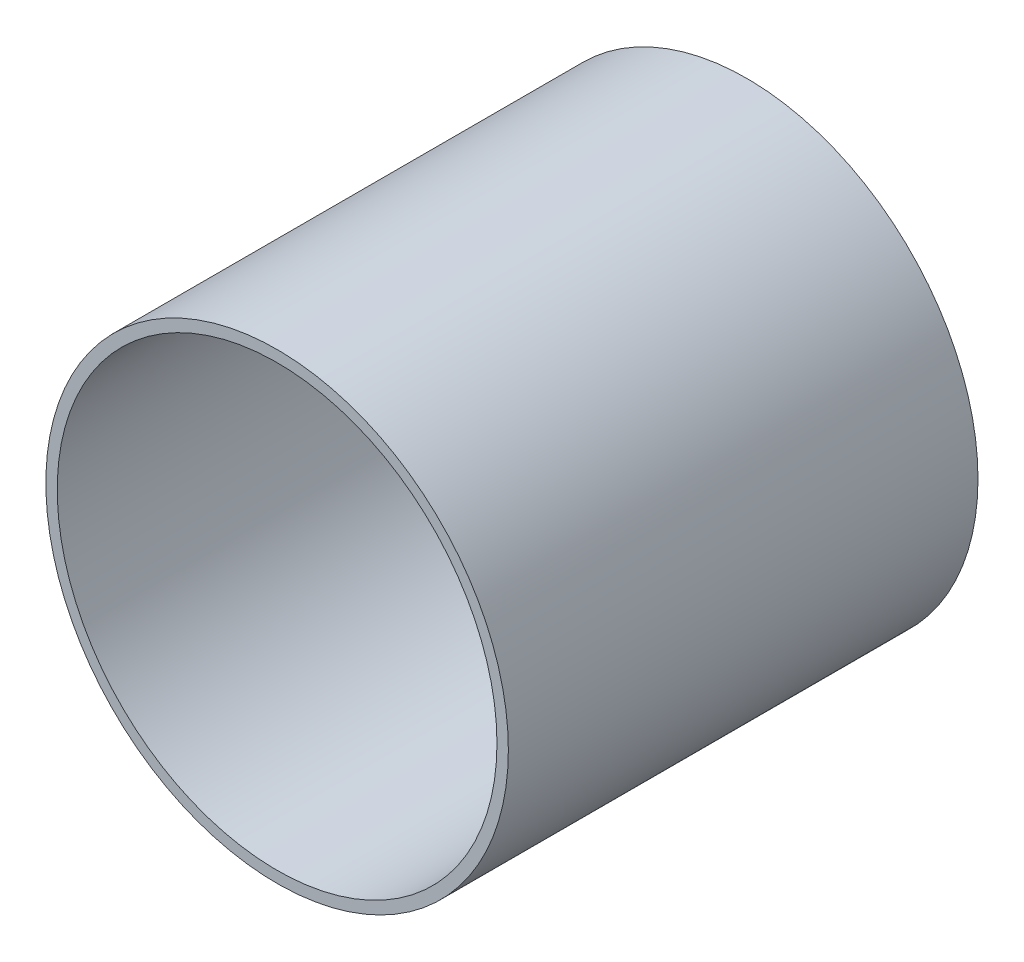
from build123d import *

# Parameters (mm, degrees)
SKETCH1_R           = 162.5
SKETCH1_R_2         = 154.5
BOSS_EXTRUDE1_DEPTH = 330


with BuildPart() as part:
    # Sketch1 → Boss-Extrude1 (new body)
    with BuildSketch(Plane.XY):
        Circle(SKETCH1_R)
        Circle(SKETCH1_R_2, mode=Mode.SUBTRACT)
    extrude(amount=BOSS_EXTRUDE1_DEPTH)


solid = part.part
